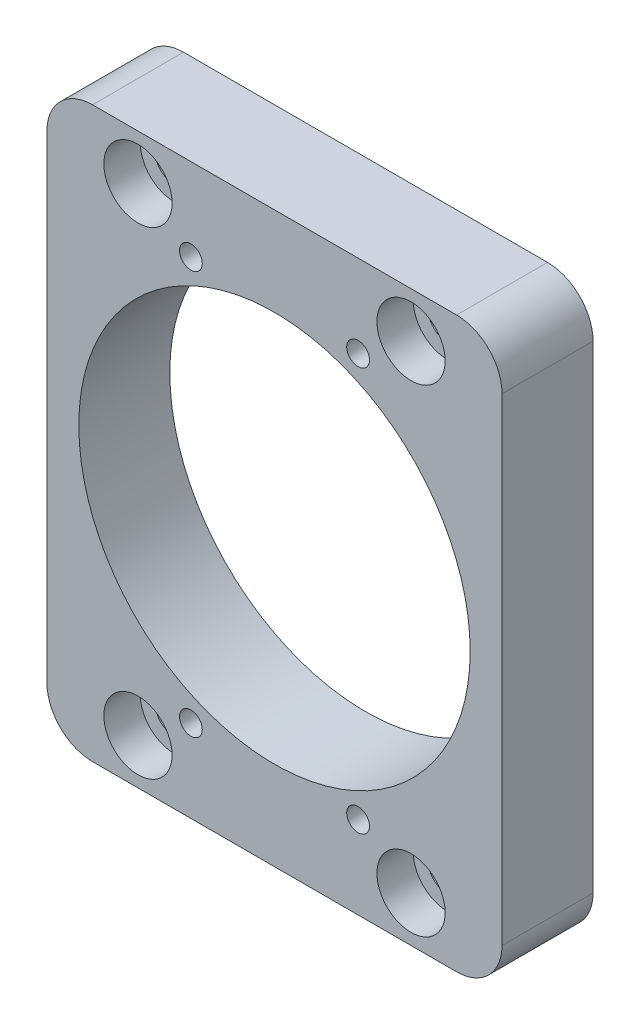
SolidWorks part; units mm, degrees
ref_plane "前视基准面" through (0, 0, 0) normal (0, 0, 1) x (1, 0, 0)
ref_plane "上视基准面" through (0, 0, 0) normal (0, 1, 0) x (1, 0, 0)
ref_plane "右视基准面" through (0, 0, 0) normal (1, 0, 0) x (0, 0, -1)
sketch "草图1" plane through (0, 0, 0) normal (0, 0, 1) x (1, 0, 0)
  line L1 (-50, 62.5) -> (50, 62.5)
  line L2 (-50, 62.5) -> (-50, -62.5)
  line L3 (-50, -62.5) -> (50, -62.5)
  line L4 (50, 62.5) -> (50, -62.5)
  line L5 (-50, 62.5) -> (50, -62.5) construction
  line L6 (-50, -62.5) -> (50, 62.5) construction
  point P0 (0, 0)
  dimension "D1" = 100
  dimension "D2" = 125
extrude "凸台-拉伸1" add sketch "草图1" along normal blind 20 contours L1 L4 L3 L2
hole_wizard "M8 六角凹头螺钉的柱形沉头孔1" positions "草图3" profile "草图2" counterbore size "M8" standard "ISO" end condition through all
sketch "草图3" plane through (0, 0, 20) normal (0, 0, 1) x (1, 0, 0)
  line L0 (-50, -62.5) -> (50, -62.5) construction
  point P0 (-30, -52.5)
  point P2 (30, -52.5)
  dimension "D1" = 60
  dimension "D2" = 30
  dimension "D3" = 10
sketch "草图2" plane through (-30, -52.5, 20) normal (1, 0, 0) x (0, -1, 0)
  line L0 (0, 0) -> (0, 20)
  line L1 (0, 20) -> (4.25, 20)
  line L3 (4.25, 20) -> (4.25, 8)
  line L4 (4.25, 8) -> (7.5, 8)
  line L5 (7.5, 8) -> (7.5, 0)
  line L7 (7.5, 0) -> (0, 0)
  line L11 (0, -6.35) -> (0, 107.95) construction
  dimension "通孔孔直径" = 8.5
  dimension "通孔孔深度" = 20
  dimension "柱形沉头孔直径" = 15
  dimension "柱形沉头孔深度" = 8
sketch "草图4" plane through (0, 0, 20) normal (0, 0, 1) x (1, 0, 0)
  circle A0 centre (0, 0) radius 43
  dimension "D1" = 86
extrude "切除-拉伸1" cut sketch "草图4" against normal through all
hole_wizard "M6 螺纹孔1" positions "草图11" profile "草图10" tap size "M6" standard "ISO" end condition through all
sketch "草图11" plane through (0, 0, 20) normal (0, 0, 1) x (1, 0, 0)
  line L0 (-18.3688, 44.3462) -> (0, 0)
  line L1 (0, 0) -> (18.3688, 44.3462)
  line L3 (0, 0) -> (0, 48)
  circle A0 centre (0, 0) radius 48
  point P4 (-18.3688, 44.3462)
  point P7 (18.3688, 44.3462)
  dimension "D1" = 96
  dimension "D2" = 45
  dimension "D3" = 22.5
sketch "草图10" plane through (-18.3688, 44.3462, 20) normal (1, 0, 0) x (0, -1, 0)
  line L0 (0, 0) -> (0, 20)
  line L1 (0, 20) -> (2.5, 20)
  line L2 (2.5, 20) -> (2.5, 0)
  line L5 (2.5, 0) -> (0, 0)
  line L11 (0, -6.35) -> (0, 107.95) construction
  dimension "通孔螺纹孔钻头直径" = 5
  dimension "通孔螺纹孔钻头深度" = 20
cosmetic thread "孔螺蚊线1" parameters "D2"=6
cosmetic thread "孔螺蚊线2" parameters "D2"=6
mirror "镜向2" about plane through (0, 0, 0) normal (0, 1, 0) of "M8 六角凹头螺钉的柱形沉头孔1", "M6 螺纹孔1"
fillet "圆角1" radius 10 4 edges at (50, 62.5, 10) (50, -62.5, 10) (-50, -62.5, 10) (-50, 62.5, 10)
